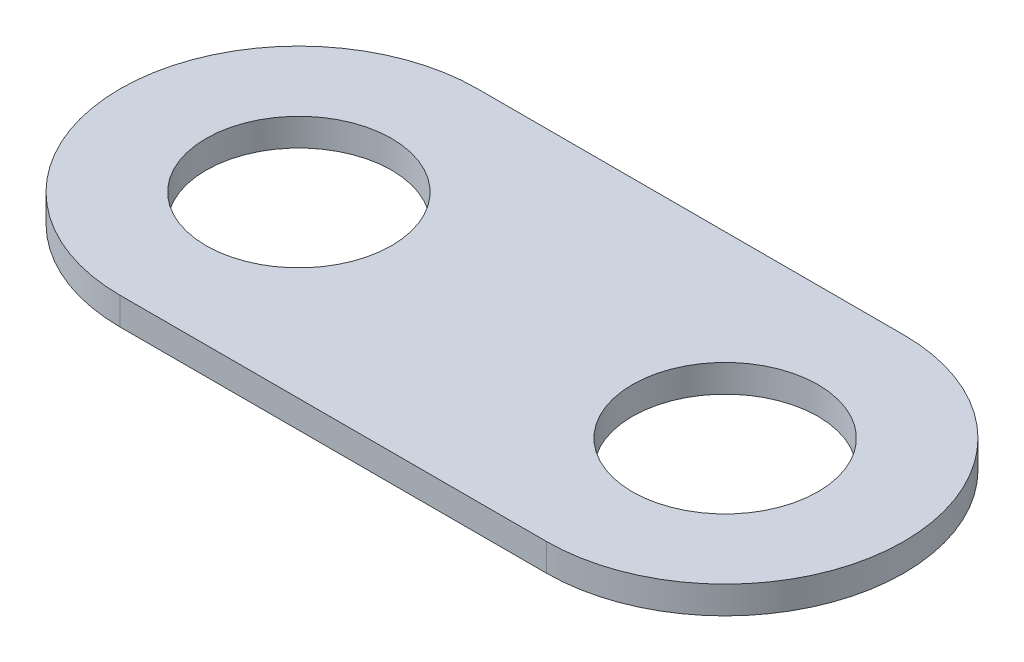
from build123d import *

# Parameters (mm, degrees)
SKETCH1_R      = 13.5
EXTRUDE1_DEPTH = 2


with BuildPart() as part:
    # Sketch1 → Extrude1 (new, symmetric)
    with BuildSketch(Plane(origin=(0, 0, 0), x_dir=(1, 0, 0), z_dir=(0, 1, 0))):
        with BuildLine():
            Line((-62, 26), (0, 26))
            ThreePointArc((0, 26), (26, 0), (0, -26))
            Line((0, -26), (-62, -26))
            ThreePointArc((-62, -26), (-88, 0), (-62, 26))
        make_face()
        with Locations(Location((0, 0, 0), (0, 0, 270))):
            Circle(SKETCH1_R, mode=Mode.SUBTRACT)
        with Locations(Location((-62, 0, 0), (0, 0, 270))):
            Circle(SKETCH1_R, mode=Mode.SUBTRACT)
    extrude(amount=EXTRUDE1_DEPTH, both=True)


solid = part.part
